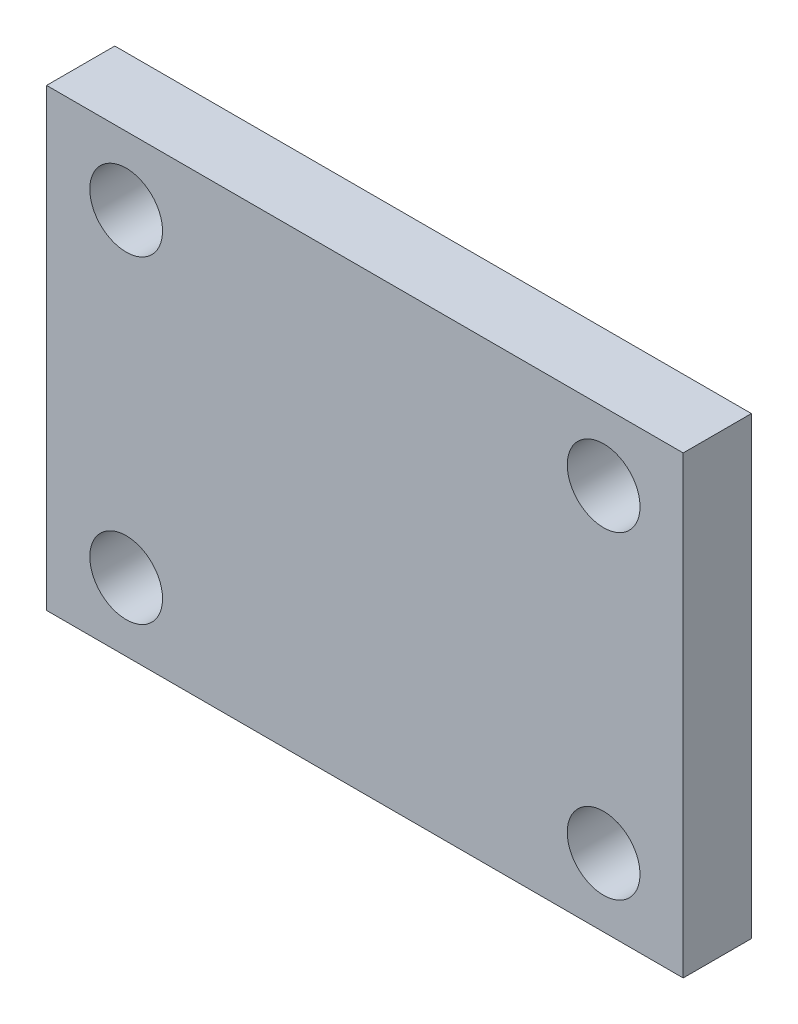
SolidWorks part; units mm, degrees
ref_plane "Front Plane" through (0, 0, 0) normal (0, 0, 1) x (1, 0, 0)
ref_plane "Top Plane" through (0, 0, 0) normal (0, 1, 0) x (1, 0, 0)
ref_plane "Right Plane" through (0, 0, 0) normal (1, 0, 0) x (0, 0, -1)
other "Configuration Table"
sketch "Sketch1" plane through (0, 0, 0) normal (0, 0, 1) x (1, 0, 0)
  line L0 (0, 0) -> (0, 50000) construction
  line L1 (14, 10) -> (-14, 10)
  line L2 (14, 10) -> (14, -10)
  line L3 (14, -10) -> (-14, -10)
  line L4 (-14, 10) -> (-14, -10)
  line L5 (14, 10) -> (-14, -10) construction
  line L6 (14, -10) -> (-14, 10) construction
  line L7 (10.5, -7) -> (-10.5, -7) construction
  line L8 (10.5, -7) -> (10.5, 7) construction
  line L9 (10.5, 7) -> (-10.5, 7) construction
  line L10 (-10.5, -7) -> (-10.5, 7) construction
  line L11 (10.5, -7) -> (-10.5, 7) construction
  line L12 (10.5, 7) -> (-10.5, -7) construction
  line L13 (0, 0) -> (50000, 0) construction
  circle A0 centre (10.5, 7) radius 1.6
  circle A1 centre (-10.5, 7) radius 1.6
  circle A2 centre (10.5, -7) radius 1.6
  circle A3 centre (-10.5, -7) radius 1.6
  point P0 (0, 0)
  point P6 (0, 0)
  dimension "D5" = 3.2
  dimension "D1" = 28
  dimension "D2" = 20
  dimension "D3" = 21
  dimension "D4" = 14
extrude "Boss-Extrude1" add sketch "Sketch1" along normal mid plane 3
